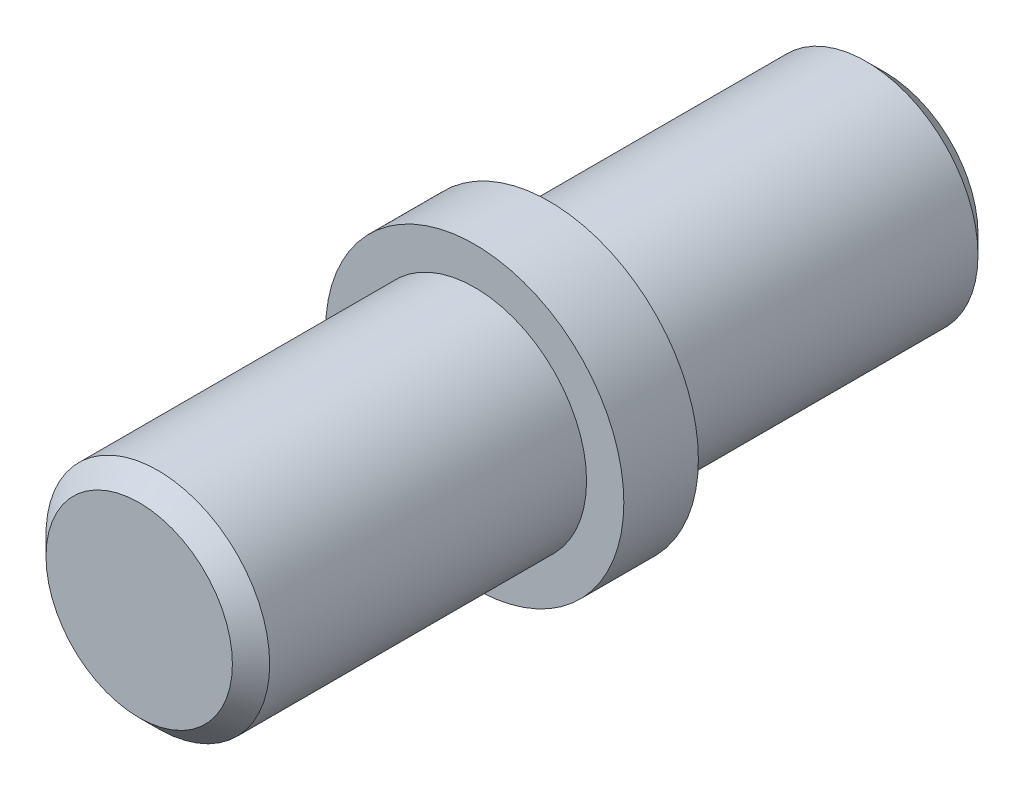
from build123d import *

# Parameters (mm, degrees)
SKETCH_1_R      = 4
EXTRUDE_1_DEPTH = 1
SKETCH_2_R      = 3
EXTRUDE_2_DEPTH = 9
CHAMFER_1_SIZE  = 0.5


with BuildPart() as part:
    # 草图1 → 凸台-拉伸1 (new, symmetric)
    with BuildSketch(Plane.XY):
        Circle(SKETCH_1_R)
    extrude(amount=EXTRUDE_1_DEPTH, both=True)

    # 草图2 → 凸台-拉伸2 (add)
    with BuildSketch(Plane.XY.offset(1)):
        Circle(SKETCH_2_R)
    extrude_2 = extrude(amount=EXTRUDE_2_DEPTH)

    # 镜向5: 凸台-拉伸2 across plane
    add(extrude_2.mirror(Plane.XY))

    # 倒角1
    chamfer_1_edges = [part.edges().sort_by_distance(p)[0] for p in [
        (-3, 0, -10),
        (-3, 0, 10),
    ]]
    chamfer(chamfer_1_edges, length=CHAMFER_1_SIZE)


solid = part.part
